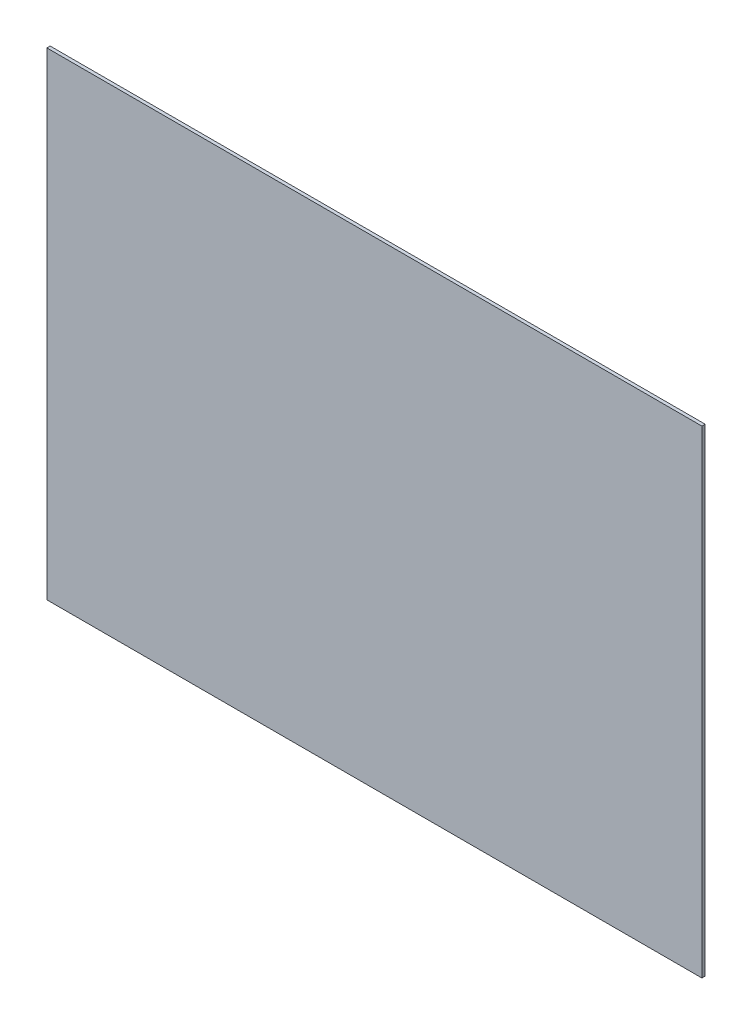
from build123d import *

# Parameters (mm, degrees)
SKETCH_1_W      = 999
SKETCH_1_H      = 729
EXTRUDE_1_DEPTH = 5


with BuildPart() as part:
    # 草图1 → 凸台-拉伸1 (new body)
    with BuildSketch(Plane.XY):
        Rectangle(SKETCH_1_W, SKETCH_1_H)
    extrude(amount=EXTRUDE_1_DEPTH)


solid = part.part
